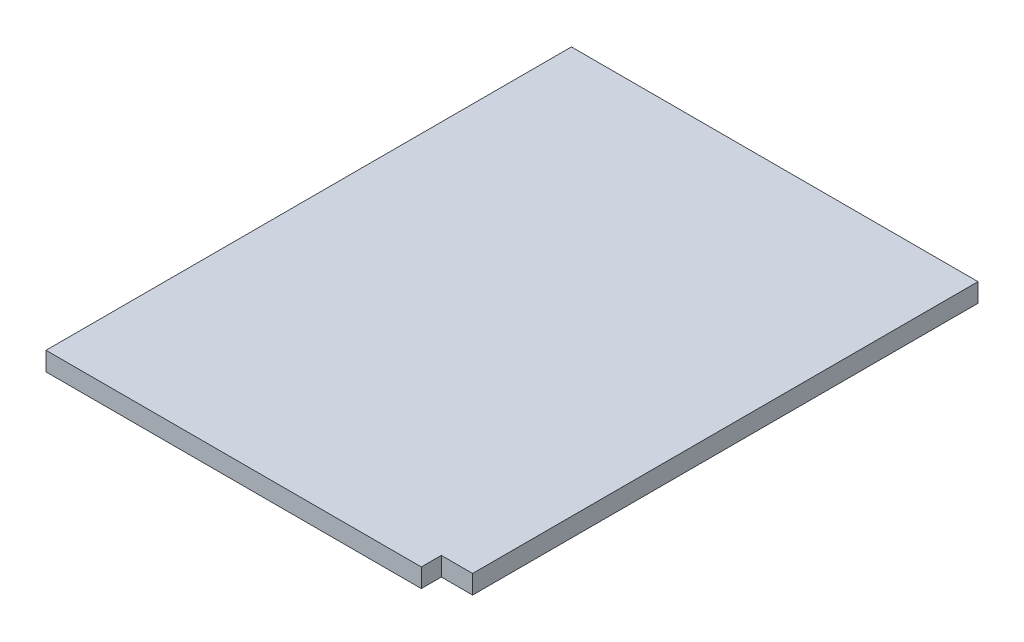
SolidWorks part; units mm, degrees
ref_plane "Front Plane" through (0, 0, 0) normal (0, 0, 1) x (1, 0, 0)
ref_plane "Top Plane" through (0, 0, 0) normal (0, 1, 0) x (1, 0, 0)
ref_plane "Right Plane" through (0, 0, 0) normal (1, 0, 0) x (0, 0, -1)
ref_plane "Plane1" through (0, 0, 0) normal (0, -1, 0) x (1, 0, 0)
sketch "Sketch1" plane through (0, 0, 0) normal (0, -1, 0) x (1, 0, 0)
  line L0 (300, 420) -> (0, 420)
  line L1 (0, 420) -> (0, 0)
  line L2 (0, 0) -> (325, 0)
  line L3 (325, 0) -> (325, 404)
  line L4 (325, 404) -> (300, 404)
  line L5 (300, 404) -> (300, 420)
extrude "Boss-Extrude1" add sketch "Sketch1" against normal blind 15
